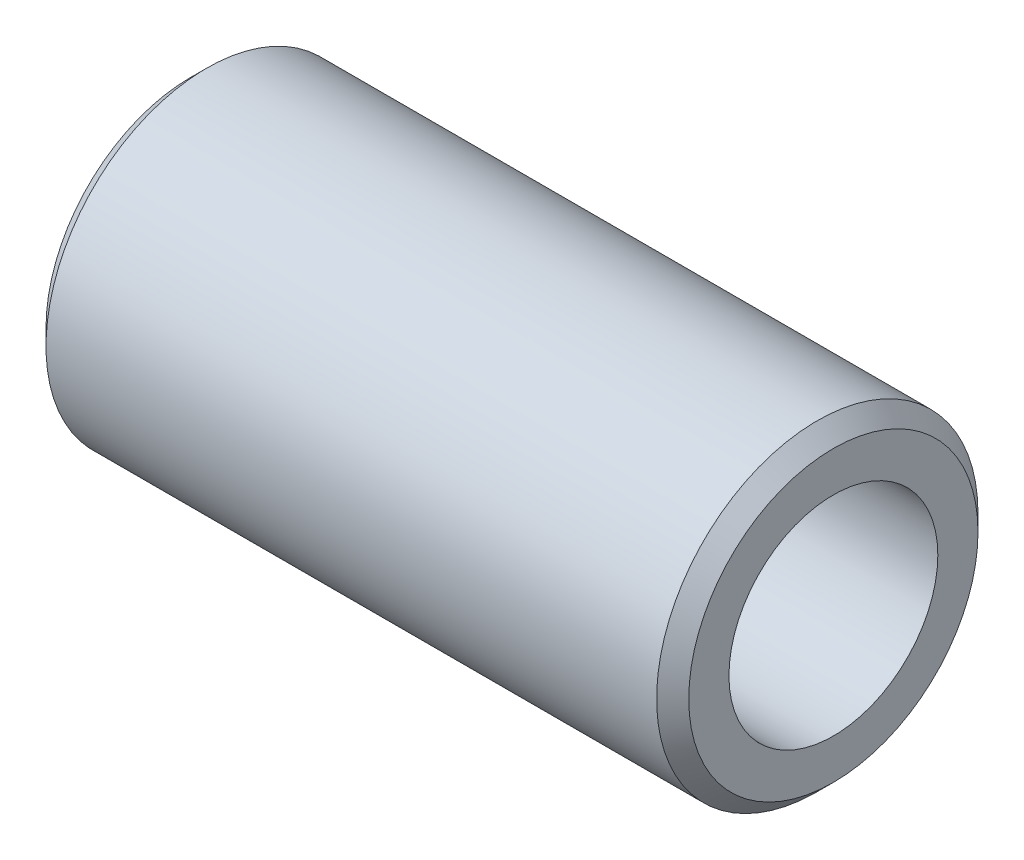
from build123d import *

# Parameters (mm, degrees)
SKETCH_1_R          = 5
EXTRUDE_1_DEPTH     = 20
CHAMFER_1_SIZE      = 0.5
SKETCH_2_R          = 3.25
CUT_EXTRUDE_1_DEPTH = 22.213203436


with BuildPart() as part:
    # 草图1 → 凸台-拉伸1 (new body)
    with BuildSketch(Plane(origin=(0, 0, 0), x_dir=(0, 0, -1), z_dir=(1, 0, 0))):
        Circle(SKETCH_1_R)
    extrude(amount=EXTRUDE_1_DEPTH)

    # 倒角1
    chamfer_1_edges = [part.edges().sort_by_distance(p)[0] for p in [
        (0, 0, 5),
        (20, 0, 5),
    ]]
    chamfer(chamfer_1_edges, length=CHAMFER_1_SIZE)

    # 草图2 → 切除-拉伸1 (cut, through all)
    with BuildSketch(Plane.ZY):
        Circle(SKETCH_2_R)
    extrude(amount=-CUT_EXTRUDE_1_DEPTH, mode=Mode.SUBTRACT)


solid = part.part
